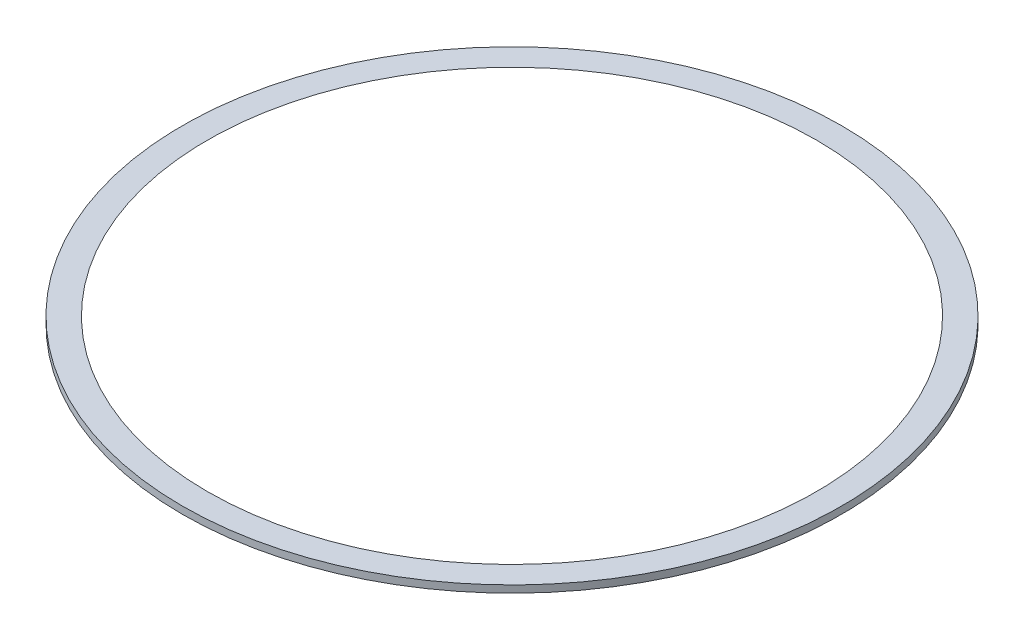
from build123d import *


with BuildPart() as part:
    # Sketch1 → Revolve1 (revolve)
    with BuildSketch(Plane.XY, mode=Mode.PRIVATE) as revolve1_sk:
        Polygon((-170, 4), (-184, 4), (-184, 0), (-176, 0), align=None)
    revolve(revolve1_sk.sketch.rotate(Axis((0, 23.75820198, 0), (0, 1, 0)), 270), axis=Axis((0, 23.75820198, 0), (0, 1, 0)))


solid = part.part
